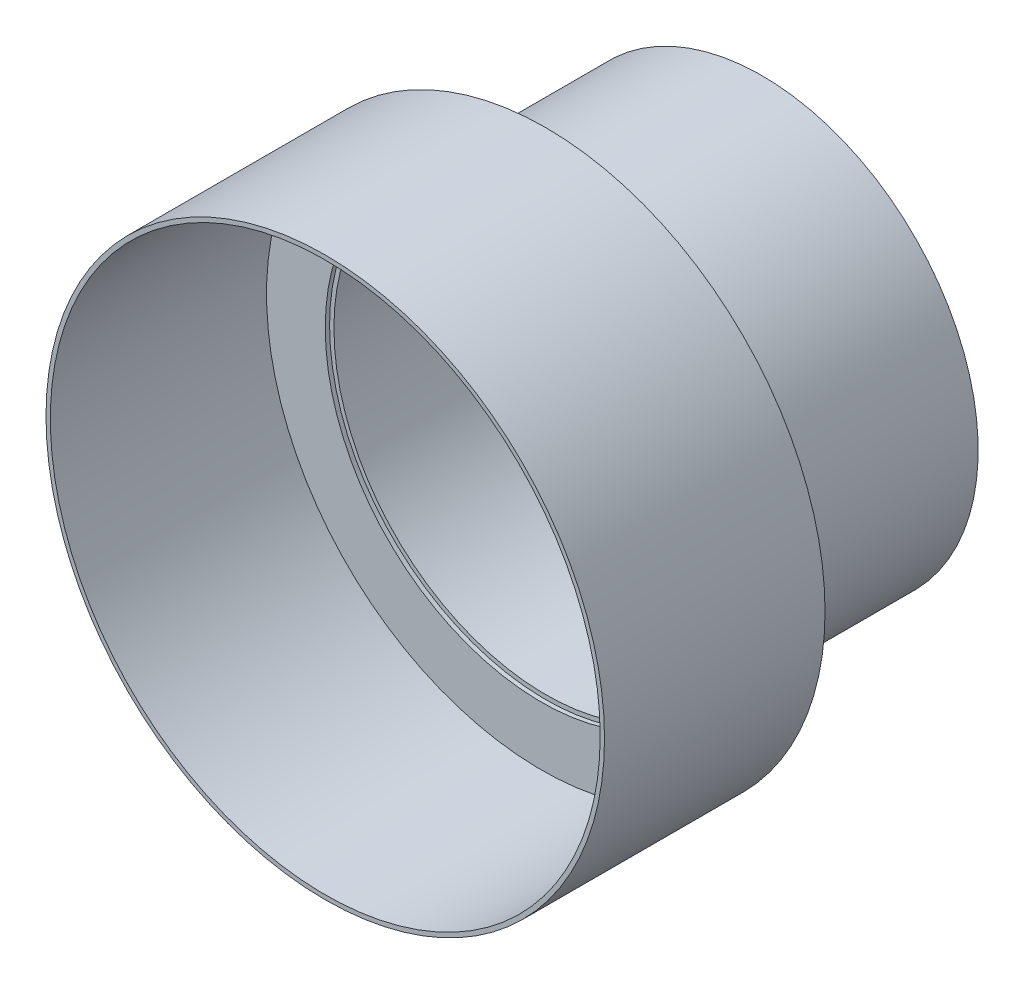
from build123d import *

# Parameters (mm, degrees)
SKETCH1_R           = 77.5
SKETCH1_R_2         = 76.3
BOSS_EXTRUDE1_DEPTH = 60
BOSS_EXTRUDE2_START = 1.2
SKETCH2_R           = 77.5
SKETCH2_R_2         = 60
BOSS_EXTRUDE2_DEPTH = 1.2
SKETCH3_R           = 60
SKETCH3_R_2         = 58.8
BOSS_EXTRUDE3_DEPTH = 60


with BuildPart() as part:
    # Sketch1 → Boss-Extrude1 (new body)
    with BuildSketch(Plane.XY):
        Circle(SKETCH1_R)
        Circle(SKETCH1_R_2, mode=Mode.SUBTRACT)
    extrude(amount=BOSS_EXTRUDE1_DEPTH)

    # Sketch2 → Boss-Extrude2 (add)
    with BuildSketch(Plane(origin=(0, 0, 0), x_dir=(-1, 0, 0), z_dir=(0, 0, -1)).offset(BOSS_EXTRUDE2_START)):
        Circle(SKETCH2_R)
        Circle(SKETCH2_R_2, mode=Mode.SUBTRACT)
    extrude(amount=-BOSS_EXTRUDE2_DEPTH)


with BuildPart() as body_2:
    # Sketch3 → Boss-Extrude3 (new body)
    with BuildSketch(Plane(origin=(0, 0, -1.2), x_dir=(-1, 0, 0), z_dir=(0, 0, -1))):
        Circle(SKETCH3_R)
        Circle(SKETCH3_R_2, mode=Mode.SUBTRACT)
    extrude(amount=BOSS_EXTRUDE3_DEPTH)


solid = Compound([part.part, body_2.part])
